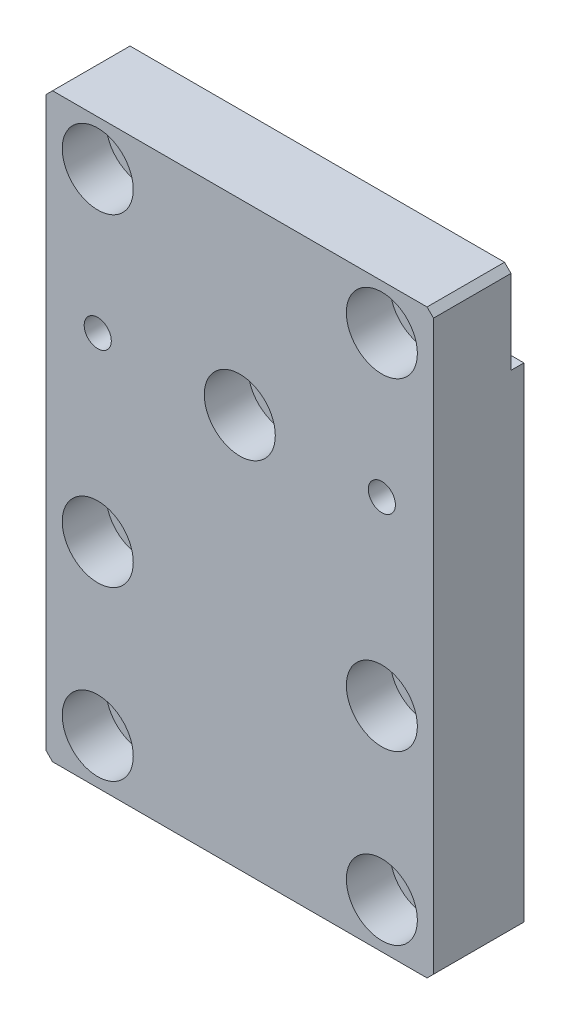
from build123d import *

# Parameters (mm, degrees)
SKETCH1_W                                            = 60
SKETCH1_H                                            = 90
BOSS_EXTRUDE1_DEPTH                                  = 7
SKETCH2_W                                            = 60
SKETCH2_H                                            = 14
CUT_EXTRUDE1_DEPTH                                   = 2
HOLE_SIZE_PER_SOCKET_HEAD_CAP_SCREW_TYPE_D           = 6.6
HOLE_SIZE_PER_SOCKET_HEAD_CAP_SCREW_TYPE_CBORE_D     = 11
HOLE_SIZE_PER_SOCKET_HEAD_CAP_SCREW_TYPE_CBORE_DEPTH = 6.8
CHAMFER1_SIZE                                        = 1
M5_TAPPED_HOLE1_D                                    = 4.2


with BuildPart() as part:
    # Sketch1 → Boss-Extrude1 (new, symmetric)
    with BuildSketch(Plane.XY):
        Rectangle(SKETCH1_W, SKETCH1_H)
    extrude(amount=BOSS_EXTRUDE1_DEPTH, both=True)

    # Sketch2 → Cut-Extrude1 (cut)
    with BuildSketch(Plane(origin=(0, 0, -7), x_dir=(-1, 0, 0), z_dir=(0, 0, -1))):
        with Locations((0, 38)):
            Rectangle(SKETCH2_W, SKETCH2_H)
    extrude(amount=-CUT_EXTRUDE1_DEPTH, mode=Mode.SUBTRACT)

    # Hole Size per Socket Head Cap Screw Type1 (through all)
    with Locations(Plane.XY.offset(7)):
        with Locations((0, 16), (-22, 38), (22, 38), (-22, -12), (22, -38), (-22, -38), (22, -12)):
            CounterBoreHole(HOLE_SIZE_PER_SOCKET_HEAD_CAP_SCREW_TYPE_D / 2, HOLE_SIZE_PER_SOCKET_HEAD_CAP_SCREW_TYPE_CBORE_D / 2, HOLE_SIZE_PER_SOCKET_HEAD_CAP_SCREW_TYPE_CBORE_DEPTH)

    # Chamfer1
    chamfer1_edges = [part.edges().sort_by_distance(p)[0] for p in [
        (30, -45, 0),
        (-30, -45, 0),
        (-30, 45, 1),
        (30, 45, 1),
    ]]
    chamfer(chamfer1_edges, length=CHAMFER1_SIZE)

    # M5 Tapped Hole1 (through all)
    with Locations(Plane.XY.offset(7)):
        with Locations((22, 16), (-22, 16)):
            Hole(M5_TAPPED_HOLE1_D / 2)


solid = part.part
